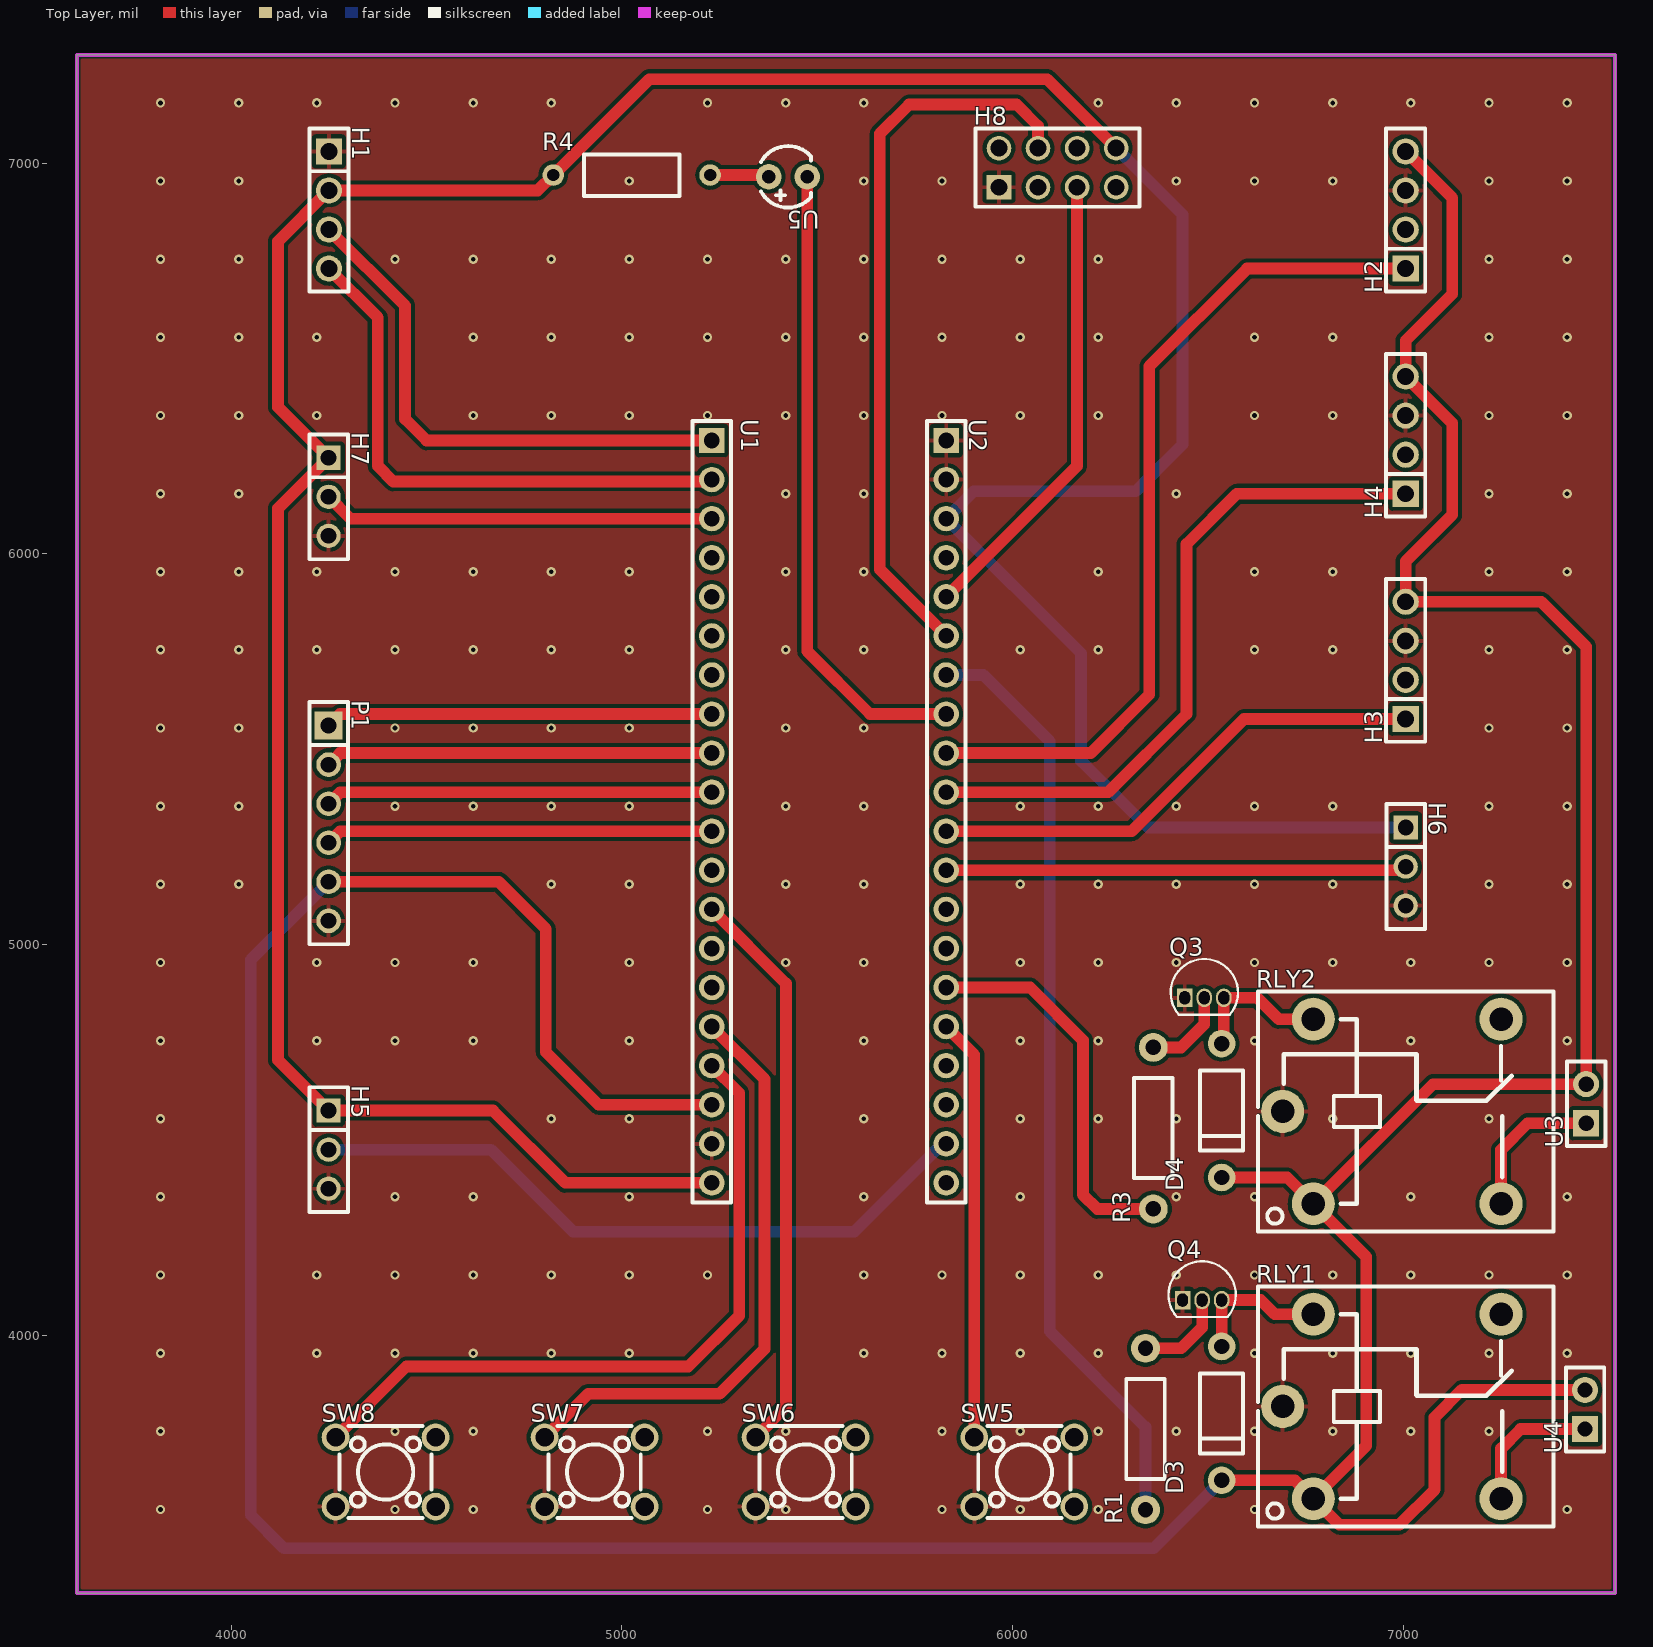
[diagram p0: Top Layer view]
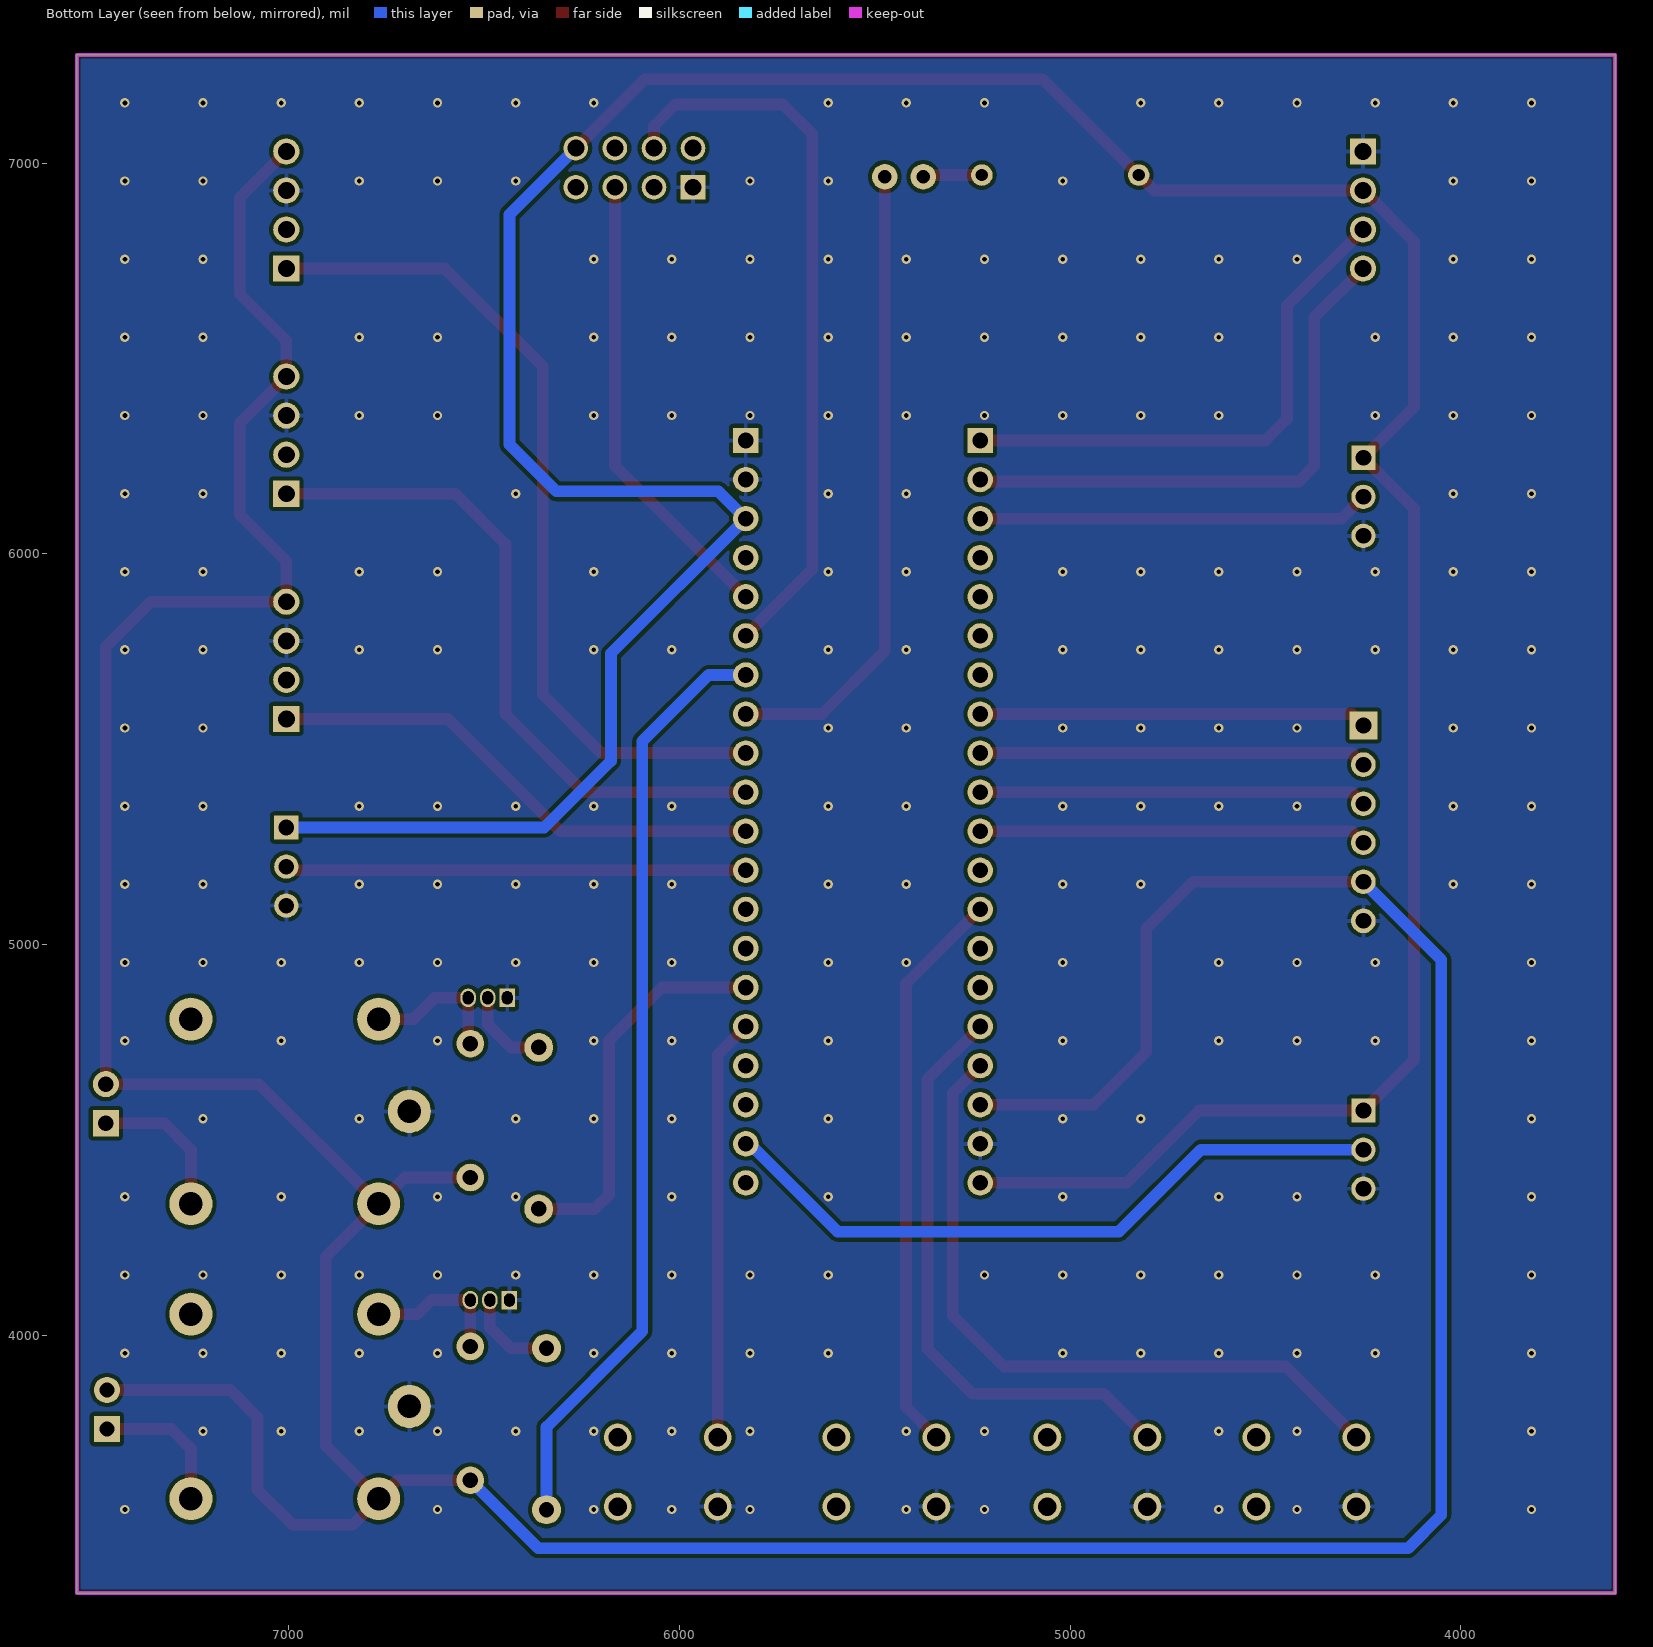
[diagram p1: Bottom Layer view, seen from below]
# Altium PCB MISC51563.pcbdoc
Units mil, origin at the board's own origin, x right, y up, seen from the top; angles counter-clockwise.
Board outline 3937.01 x 3937.01 mil, 2 copper layers (Top Layer, Bottom Layer), stack 62.206 mil thick; 27 components, 38 nets, 127 pads, 246 vias.

## Layer stack, top to bottom
Top Solder Mask Layer: solder mask 0.394, Dk 3.3
Top Layer: signal copper 1.379
Dielectric1: surface 59.449, FR4, Dk 4.5
Bottom Layer: signal copper 1.378
Bottom Solder Mask Layer: solder mask 0.394, Dk 3.3

## Board outline
3605,7277.01 3605,3340 7542.01,3340 7542.01,7277.01

## Design rules (kind name [scope] priority, off if disabled: settings)
BoardOutlineClearance copperThickness2oz_1 [All] p2 off: genericclearance=7.99 ignorepadtopadclearanceinfootprint=FALSE except(0: Arc-SplitContinuation Track-SplitContinuation SMDPad-SplitContinuation THPad-SplitContinuation Via-SplitContinuation Fill-SplitContinuation Region-SplitContinuation Poly-SplitContinuation Text-SplitContinuation Hole-SplitContinuation; 5.98: Arc-CutoutEdge SMDPad-CutoutEdge THPad-CutoutEdge Via-CutoutEdge Fill-CutoutEdge Region-CutoutEdge Text-CutoutEdge; 6.93: Hole-OutlineEdge Hole-CutoutEdge; 10: Poly-OutlineEdge Poly-CutoutEdge; 11.81: Arc-OutlineEdge Track-OutlineEdge SMDPad-OutlineEdge THPad-OutlineEdge Via-OutlineEdge Fill-OutlineEdge Region-OutlineEdge Text-OutlineEdge Track-CutoutEdge)
BoardOutlineClearance Plane_innerPlane_1 [All] p4 off: genericclearance=4.02 ignorepadtopadclearanceinfootprint=FALSE except(0: Arc-SplitContinuation Track-SplitContinuation SMDPad-SplitContinuation THPad-SplitContinuation Via-SplitContinuation Fill-SplitContinuation Region-SplitContinuation Poly-SplitContinuation Text-SplitContinuation Hole-SplitContinuation; 6: SMDPad-CutoutEdge THPad-CutoutEdge Via-CutoutEdge Fill-CutoutEdge Region-CutoutEdge Text-CutoutEdge; 6.93: Hole-OutlineEdge Hole-CutoutEdge; 10: Poly-OutlineEdge Poly-CutoutEdge; 11.8: Arc-OutlineEdge Track-OutlineEdge SMDPad-OutlineEdge THPad-OutlineEdge Via-OutlineEdge Fill-OutlineEdge Region-OutlineEdge Text-OutlineEdge; 11.81: Arc-CutoutEdge Track-CutoutEdge)
BoardOutlineClearance Copper_copperRegion_1 [All] p6 off: genericclearance=4.02 ignorepadtopadclearanceinfootprint=FALSE except(0: Arc-SplitContinuation Track-SplitContinuation SMDPad-SplitContinuation THPad-SplitContinuation Via-SplitContinuation Fill-SplitContinuation Region-SplitContinuation Poly-SplitContinuation Text-SplitContinuation Hole-SplitContinuation; 6: SMDPad-CutoutEdge THPad-CutoutEdge Via-CutoutEdge Fill-CutoutEdge Region-CutoutEdge Text-CutoutEdge; 6.93: Hole-OutlineEdge Hole-CutoutEdge; 10: Poly-OutlineEdge Poly-CutoutEdge; 11.8: Arc-OutlineEdge Track-OutlineEdge SMDPad-OutlineEdge THPad-OutlineEdge Via-OutlineEdge Fill-OutlineEdge Region-OutlineEdge Text-OutlineEdge; 11.81: Arc-CutoutEdge Track-CutoutEdge)
BoardOutlineClearance copperThickness1oz_1 [All] p8: genericclearance=4.02 ignorepadtopadclearanceinfootprint=FALSE except(0: Arc-SplitContinuation Track-SplitContinuation SMDPad-SplitContinuation THPad-SplitContinuation Via-SplitContinuation Fill-SplitContinuation Region-SplitContinuation Poly-SplitContinuation Text-SplitContinuation Hole-SplitContinuation; 6: SMDPad-CutoutEdge THPad-CutoutEdge Via-CutoutEdge Fill-CutoutEdge Region-CutoutEdge Text-CutoutEdge; 6.93: Hole-OutlineEdge Hole-CutoutEdge; 10: Poly-OutlineEdge Poly-CutoutEdge; 11.8: Arc-OutlineEdge Track-OutlineEdge SMDPad-OutlineEdge THPad-OutlineEdge Via-OutlineEdge Fill-OutlineEdge Region-OutlineEdge Text-OutlineEdge; 11.81: Arc-CutoutEdge Track-CutoutEdge)
Clearance copperThickness2oz [All] p1 off: gap=7.99 ignorepadtopadclearanceinfootprint=FALSE except(5.98: SMDPad-Track SMDPad-SMDPad THPad-Track SMDPad-THPad THPad-THPad Track-Via SMDPad-Via THPad-Via Via-Via Fill-Track Region-Track Fill-SMDPad Region-SMDPad Fill-THPad Region-THPad Fill-Via Region-Via Fill-Fill Fill-Region Region-Region Arc-Track Arc-SMDPad Arc-THPad Arc-Via Fill-Arc Region-Arc Arc-Arc Text-Track SMDPad-Text Text-THPad Text-Via Fill-Text Region-Text Arc-Text Text-Text; 6.93: Hole-Track Hole-SMDPad Hole-THPad Hole-Via Fill-Hole Region-Hole Hole-Arc Hole-Text; 10: Poly-Track Poly-SMDPad Poly-THPad Poly-Via Poly-Fill Poly-Region Poly-Poly Poly-Arc Poly-Text Poly-Hole)
Clearance Plane_innerPlane [All] p3 off: gap=4.02 ignorepadtopadclearanceinfootprint=FALSE except(5.98: SMDPad-Track SMDPad-SMDPad THPad-Track SMDPad-THPad THPad-THPad Track-Via SMDPad-Via THPad-Via Via-Via Fill-Track Region-Track Fill-SMDPad Region-SMDPad Fill-THPad Region-THPad Fill-Via Region-Via Fill-Fill Fill-Region Region-Region; 6: Arc-Track Arc-SMDPad Arc-THPad Arc-Via Fill-Arc Region-Arc Arc-Arc Text-Track SMDPad-Text Text-THPad Text-Via Fill-Text Region-Text Arc-Text Text-Text; 6.93: Hole-Track Hole-SMDPad Hole-THPad Hole-Via Fill-Hole Region-Hole Hole-Arc Hole-Text; 10: Poly-Track Poly-SMDPad Poly-THPad Poly-Via Poly-Fill Poly-Region Poly-Poly Poly-Arc Poly-Text Poly-Hole)
Clearance Copper_copperRegion [All] p5 off: gap=4.02 ignorepadtopadclearanceinfootprint=FALSE except(5.98: SMDPad-Track SMDPad-SMDPad THPad-Track SMDPad-THPad THPad-THPad Track-Via SMDPad-Via THPad-Via Via-Via Fill-Track Region-Track Fill-SMDPad Region-SMDPad Fill-THPad Region-THPad Fill-Via Region-Via Fill-Fill Fill-Region Region-Region; 6: Arc-Track Arc-SMDPad Arc-THPad Arc-Via Fill-Arc Region-Arc Arc-Arc Text-Track SMDPad-Text Text-THPad Text-Via Fill-Text Region-Text Arc-Text Text-Text; 6.93: Hole-Track Hole-SMDPad Hole-THPad Hole-Via Fill-Hole Region-Hole Hole-Arc Hole-Text; 10: Poly-Track Poly-SMDPad Poly-THPad Poly-Via Poly-Fill Poly-Region Poly-Poly Poly-Arc Poly-Text Poly-Hole)
Clearance copperThickness1oz [All] p7: gap=4.02 ignorepadtopadclearanceinfootprint=FALSE except(5.98: SMDPad-Track SMDPad-SMDPad THPad-Track SMDPad-THPad THPad-THPad Track-Via SMDPad-Via THPad-Via Via-Via Fill-Track Region-Track Fill-SMDPad Region-SMDPad Fill-THPad Region-THPad Fill-Via Region-Via Fill-Fill Fill-Region Region-Region; 6: Arc-Track Arc-SMDPad Arc-THPad Arc-Via Fill-Arc Region-Arc Arc-Arc Text-Track SMDPad-Text Text-THPad Text-Via Fill-Text Region-Text Arc-Text Text-Text; 6.93: Hole-Track Hole-SMDPad Hole-THPad Hole-Via Fill-Hole Region-Hole Hole-Arc Hole-Text; 10: Poly-Track Poly-SMDPad Poly-THPad Poly-Via Poly-Fill Poly-Region Poly-Poly Poly-Arc Poly-Text Poly-Hole)
DiffPairsRouting differentialPair [All] p1: maxlimit=6 minlimit=6 mostfreqgap=6 toplayer_minwidth=5 toplayer_prefwidth=10 toplayer_maxwidth=100 toplayer_mingap=6 toplayer_prefgap=6 toplayer_maxgap=6 bottomlayer_minwidth=5 bottomlayer_prefwidth=10 bottomlayer_maxwidth=100 bottomlayer_mingap=6 bottomlayer_prefgap=6 bottomlayer_maxgap=6 maxuncoupledlength=10
HoleToHoleClearance otherClearance [All] p1: gap=11.81 allowstackedmicrovias=TRUE
Length netLength [All] p1: minlimit=0 maxlimit=0
PasteMaskExpansion pasteMaskExpansion [All] p1: expansion=0
PlaneConnect innerPlane [All] p1: planeconnectstyle=Relief reliefexpansion=20 reliefentries=4 reliefconductorwidth=10 reliefairgap=10
PolygonConnect copperRegion [All] p1: connectstyle=Relief reliefconductorwidth=10 reliefentries=4 polygonreliefangle="90 Angle" airgapwidth=10 via.connectstyle=Relief via.reliefconductorwidth=10 via.reliefentries=4 via.polygonreliefangle="90 Angle" via.airgapwidth=10
RoutingVias viaSize [All] p1: holewidth=12.01 width=24.02 viastyle="Through Hole" minholewidth=11.81 minwidth=19.68 maxholewidth=248.03 maxwidth=393.7
SolderMaskExpansion solderMaskExpansion [IsVia] p1: expansion=-1000 istentingtop=TRUE
SolderMaskExpansion solderMaskExpansion [All] p2: expansion=2 istentingtop=FALSE
Width copperThickness2oz_2 [All] p1 off: maxlimit=100 minlimit=8 preferedwidth=10
Width copperThickness1oz_2 [All] p2: maxlimit=100 minlimit=5 preferedwidth=10

## Components (designator, comment, footprint, x,y, rotation, side; value= is the part's Value field where it differs from the comment)
D3 "1N4001" DO-41_BD2.4-L4.7-P8.70-D0.9-RD 6535,3800 r90 top
D4 "1N4001" DO-41_BD2.4-L4.7-P8.70-D0.9-RD 6535,4575 r90 top
H1 "oled" HDR-TH_4P-P2.54-V-F 4250,6880 r270 top
H2 "mq2" HDR-TH_4P-P2.54-V-F 7005.98,6880 r90 top
H3 "mq7" HDR-TH_4P-P2.54-V-F 7005.98,5727.36 r90 top
H4 "mq135" HDR-TH_4P-P2.54-V-F 7005.98,6303.68 r90 top
H5 "Buzzer" HDR-TH_3P-P2.54-V-F 4249.21,4475 r270 top
H6 "Photoresistor" HDR-TH_3P-P2.54-V-F 7005.98,5199.47 r270 top
H7 "dht22" HDR-TH_3P-P2.54-V-F 4249.21,6146.05 r270 top
H8 "esp8266" HDR-TH_8P-P2.54-V-F-R2-C4-S2.54 6115,6988.27 r0 top
P1 "uln2003" HDR-TH_6P-P2.54-V-F 4249.21,5310.52 r270 top
Q3 "S8050" TO-92-3_L4.5-W3.5-P1.27-L 6490.51,4863.59 r0 top
Q4 "S8050" TO-92-3_L4.5-W3.5-P1.27-L 6485,4090 r0 top
R1 "1kΩ" RES-TH_BD2.5-L6.5-P10.50-D0.6 6340,3760 r90 top
R3 "1kΩ" RES-TH_BD2.5-L6.5-P10.50-D0.6 6360,4530 r90 top
R4 "10kΩ" RES-TH_BD2.7-L6.2-P10.20-D0.4 5025,6969.41 r0 top
RLY1 "SRD-05VDC-SL-C" RELAY-TH_SRD-XXVDC-XL-C 6970.51,3817.75 r0 top
RLY2 "SRD-05VDC-SL-C" RELAY-TH_SRD-XXVDC-XL-C 6970.51,4572.75 r0 top
SW5 "TC-00104-050E" SW-TH_4P-L6.0-W6.0-P4.50-LS6.5 6030,3650 r0 top
SW6 "TC-00104-050E" SW-TH_4P-L6.0-W6.0-P4.50-LS6.5 5470,3650 r0 top
SW7 "TC-00104-050E" SW-TH_4P-L6.0-W6.0-P4.50-LS6.5 4930,3650 r0 top
SW8 "TC-00104-050E" SW-TH_4P-L6.0-W6.0-P4.50-LS6.5 4395,3650 r0 top
U1 "KH-2.54FH-1X20P-H8.5" HDR-TH_20P-P2.54-V-F-2 5230,5340 r270 top
U2 "KH-2.54FH-1X20P-H8.5" HDR-TH_20P-P2.54-V-F-2 5830,5340 r270 top
U3 "Humidifier" HDR-TH_2P-P2.54-V-F 7467.83,4592.75 r90 top
U4 "Fan" HDR-TH_2P-P2.54-V-F 7465,3810 r90 top
U5 "204-10SDRD/S530-A3/F182-68" LED-TH_BD4.0-P2.50-RD 5425,6965 r180 top

## Footprints (in the part's own frame and the unit in brackets; to place one, negate y for a bottom-side part, rotate by r counter-clockwise, add the part's x,y. Pads: shape width x height; smd on the part's side, far side on the other; paste and mask are expansions set on the pad)
DO-41_BD2.4-L4.7-P8.70-D0.9-RD [mm]
  round 1.8 hole 1: 1(-4.35,0) 2(4.35,0)
  silkscreen extent -2.6,-1.4 2.6,1.4
HDR-TH_2P-P2.54-V-F [mm]
  rect 1.7x1.7 hole 1: 1(-1.27,0)
  round 1.7 hole 1: 2(1.27,0)
  silkscreen extent -2.74,-1.25 2.74,1.25
HDR-TH_3P-P2.54-V-F [mil]
  rect 62x62 hole 40.16: 1(-100,0)
  round 62 hole 40.16: 2(0,0) 3(100,0)
  silkscreen extent -160,-49 160,49
HDR-TH_4P-P2.54-V-F [mm]
  rect 1.7x1.7 hole 1.1: 1(-3.81,0)
  round 1.7 hole 1.1: 2(-1.27,0) 3(1.27,0) 4(3.81,0)
  silkscreen extent -5.29,-1.27 5.29,1.27
HDR-TH_6P-P2.54-V-F [mm]
  rect 1.8x1.8 hole 1.02: 1(-6.35,0)
  round 1.6 hole 1.02: 2(-3.81,0) 3(-1.27,0) 4(1.27,0) 5(3.81,0) 6(6.35,0)
  silkscreen extent -7.87,-1.25 7.87,1.25
HDR-TH_8P-P2.54-V-F-R2-C4-S2.54 [mm]
  rect 1.6x1.6 hole 1.1: 1(-3.81,-1.27)
  round 1.6 hole 1.1: 2(-3.81,1.27) 3(-1.27,-1.27) 4(-1.27,1.27) 5(1.27,-1.27) 6(1.27,1.27) 7(3.81,-1.27) 8(3.81,1.27)
  silkscreen extent -5.33,-2.54 5.33,2.54
HDR-TH_20P-P2.54-V-F-2 [mm]
  rect 1.65x1.65 hole 1.02: 1(-24.13,0)
  round 1.65 hole 1.02: 2(-21.59,0) 3(-19.05,0) 4(-16.51,0) 5(-13.97,0) 6(-11.43,0) 7(-8.89,0) 8(-6.35,0) 9(-3.81,0) 10(-1.27,0) 11(1.27,0) 12(3.81,0) 13(6.35,0) 14(8.89,0) 15(11.43,0) 16(13.97,0) 17(16.51,0) 18(19.05,0) 19(21.59,0) 20(24.13,0)
  silkscreen extent -25.4,-1.25 25.4,1.25
LED-TH_BD4.0-P2.50-RD [mil]
  round 65 hole 35.43: 1(-49.21,0) 2(49.22,0)
  silkscreen extent -59,-79 69,79
RELAY-TH_SRD-XXVDC-XL-C [mil]
  round 110 hole 60: 1(-200.79,-236.22) 2(279.53,-236.2) 3(279.53,236.2) 4(-200.79,236.22) 5(-279.53,0)
  silkscreen extent -342,-307 413,307
RES-TH_BD2.5-L6.5-P10.50-D0.6 [mil]
  round 74 hole 39.37: 1(-206.69,0) 2(206.69,0)
  silkscreen extent -128,-49 128,49
RES-TH_BD2.7-L6.2-P10.20-D0.4 [mm]
  round 1.4 hole 0.8 copper offset 0,0: 1(-5.1,0) 2(5.1,0)
  silkscreen extent -3.1,-1.35 3.1,1.35
SW-TH_4P-L6.0-W6.0-P4.50-LS6.5 [mm]
  round 1.8 hole 1.2: 1(-3.25,2.25) 2(3.25,2.25) 3(-3.25,-2.25) 4(3.25,-2.25)
  silkscreen extent -3,-3 3,3
TO-92-3_L4.5-W3.5-P1.27-L [mm]
  rect 1x1.2 hole 0.7 slot 0.85 at 90 deg: 1(-1.27,0)
  oval 1x1.2 hole 0.7 slot 0.85 at 90 deg: 2(0,0) 3(1.27,0)
  silkscreen extent -2.19,-1.1 2.19,2.52

## Via types
v1: diameter 24.02, hole 12, Top Layer to Bottom Layer, 246 vias

## Nets (pads, with @x,y where several pads share a name; then routed paths per layer and width w, separated by ;. In a path a pad name is that pad's centre, name@x,y a point inside that pad or via, vN(x,y) a via of type N, cw(c..) or ccw(c..) an arc to the next point about the centre after c; other vN are vias at no path point)
$1N3: R4.2 U5.2 | length 151.8
  Top Layer w30: R4.2 5371.38,6969.41 U5.2
$1N5: SW7.2
$1N6: SW6.2
$1N12: RLY2.2 U3.1 | length 384.3
  Top Layer w30: RLY2.2 7250.04,4475.04 7317.75,4542.75 U3.1
$1N16: Q3.2 R3.2 | length 222.9
  Top Layer w30: R3.2 6431.69,4736.69 6490.51,4795.51 Q3.2
$1N17: D4.2 Q3.3 RLY2.4 | length 371.4
  Top Layer w30: D4.2 6540.51,4751.77 Q3.3 6626.41,4863.59 6681.03,4808.97 RLY2.4
$1N18: RLY1.2 U4.1 | length 364.1
  Top Layer w30: RLY1.2 7250.04,3710.04 7300,3760 U4.1
$1N22: Q4.2 R1.2 | length 237.1
  Top Layer w30: R1.2 6431.69,3966.69 6485,4020 Q4.2
$1N23: D3.2 Q4.3 RLY1.4 | length 368.4
  Top Layer w30: D3.2 Q4.3 6635,4090 6671.03,4053.97 RLY1.4
$1N97: SW8.2
+5V: D3.1 D4.1 H2.4 H3.4 H4.4 P1.5 RLY1.1 RLY2.1 U1.18 U3.2 U4.2 | length 11858.6
  Top Layer w30: P1.5 4684.48,5160.52 4805,5040 4805,4725 4940,4590 U1.18 ; D3.1 6722.51,3628.74 RLY1.1 ; D4.1 6702.51,4403.74 RLY2.1 ; H2.4 7125,6910.98 7125,6665 7005.98,6545.98 H4.4 7125,6334.66 7125,6100 7005.98,5980.98 H3.4 7352.64,5877.36 7467.83,5762.17 U3.2 7075.94,4642.75 RLY2.1 ; U4.2 7150,3860 7080,3790 7080,3605 6990,3515 6836.25,3515 RLY1.1 ; RLY1.1 6905,3716.82 6905,4201.25 RLY2.1
  Bottom Layer w30: P1.5 4050,4961.31 4050,3540 4135,3455 6361.26,3455 D3.1
GND: H1.1 H2.3 H3.3 H4.3 H5.3 H6.3 H7.3 H8.1 P1.6 Q3.1 Q4.1 RLY1.5 RLY2.5 SW5.3 SW6.3 SW7.3 SW8.3 U1.19 U2.1 U2.2
  other v1: 3819.1,3554.1 4419.1,3554.1 4619.1,3554.1 5219.1,3554.1 5419.1,3554.1 5819.1,3554.1 6019.1,3554.1 6219.1,3554.1 6619.1,3554.1 7419.1,3554.1 3819.1,3754.1 4419.1,3754.1 4619.1,3754.1 5219.1,3754.1 5419.1,3754.1 5819.1,3754.1 6019.1,3754.1 6219.1,3754.1 6419.1,3754.1 6619.1,3754.1 6819.1,3754.1 7019.1,3754.1 7219.1,3754.1 3819.1,3954.1 4219.1,3954.1 4419.1,3954.1 4619.1,3954.1 4819.1,3954.1 5019.1,3954.1 5619.1,3954.1 5819.1,3954.1 6019.1,3954.1 6219.1,3954.1 6619.1,3954.1 6819.1,3954.1 7019.1,3954.1 7219.1,3954.1 7419.1,3954.1 3819.1,4154.1 4219.1,4154.1 4419.1,4154.1 4619.1,4154.1 4819.1,4154.1 5019.1,4154.1 5219.1,4154.1 5619.1,4154.1 5819.1,4154.1 6019.1,4154.1 6219.1,4154.1 6419.1,4154.1 6619.1,4154.1 6819.1,4154.1 7019.1,4154.1 7219.1,4154.1 7419.1,4154.1 3819.1,4354.1 4419.1,4354.1 4619.1,4354.1 5019.1,4354.1 5619.1,4354.1 6019.1,4354.1 6419.1,4354.1 6619.1,4354.1 7019.1,4354.1 7419.1,4354.1 3819.1,4554.1 4819.1,4554.1 5019.1,4554.1 5619.1,4554.1 6019.1,4554.1 6219.1,4554.1 6419.1,4554.1 6819.1,4554.1 7219.1,4554.1 3819.1,4754.1 4219.1,4754.1 4419.1,4754.1 4619.1,4754.1 5019.1,4754.1 5619.1,4754.1 6019.1,4754.1 6219.1,4754.1 6619.1,4754.1 7019.1,4754.1 7419.1,4754.1 3819.1,4954.1 4219.1,4954.1 4419.1,4954.1 4619.1,4954.1 5019.1,4954.1 5419.1,4954.1 5619.1,4954.1 6019.1,4954.1 6219.1,4954.1 6419.1,4954.1 6619.1,4954.1 6819.1,4954.1 7019.1,4954.1 7219.1,4954.1 7419.1,4954.1 3819.1,5154.1 4019.1,5154.1 4819.1,5154.1 5019.1,5154.1 5419.1,5154.1 5619.1,5154.1 6019.1,5154.1 6219.1,5154.1 6419.1,5154.1 6619.1,5154.1 6819.1,5154.1 7219.1,5154.1 7419.1,5154.1 3819.1,5354.1 4019.1,5354.1 4419.1,5354.1 4619.1,5354.1 4819.1,5354.1 5019.1,5354.1 5419.1,5354.1 5619.1,5354.1 6019.1,5354.1 6219.1,5354.1 6419.1,5354.1 6619.1,5354.1 6819.1,5354.1 7219.1,5354.1 7419.1,5354.1 3819.1,5554.1 4019.1,5554.1 4419.1,5554.1 4619.1,5554.1 4819.1,5554.1 5019.1,5554.1 5419.1,5554.1 5619.1,5554.1 7219.1,5554.1 7419.1,5554.1 3819.1,5754.1 4019.1,5754.1 4219.1,5754.1 4419.1,5754.1 4619.1,5754.1 4819.1,5754.1 5019.1,5754.1 5419.1,5754.1 5619.1,5754.1 6019.1,5754.1 6219.1,5754.1 6619.1,5754.1 6819.1,5754.1 7219.1,5754.1 7419.1,5754.1 3819.1,5954.1 4019.1,5954.1 4219.1,5954.1 4419.1,5954.1 4619.1,5954.1 4819.1,5954.1 5019.1,5954.1 5419.1,5954.1 5619.1,5954.1 6219.1,5954.1 6619.1,5954.1 6819.1,5954.1 7219.1,5954.1 7419.1,5954.1 3819.1,6154.1 4019.1,6154.1 5419.1,6154.1 5619.1,6154.1 6419.1,6154.1 7219.1,6154.1 7419.1,6154.1 3819.1,6354.1 4019.1,6354.1 4219.1,6354.1 4619.1,6354.1 4819.1,6354.1 5019.1,6354.1 5219.1,6354.1 5419.1,6354.1 5619.1,6354.1 5819.1,6354.1 6019.1,6354.1 6219.1,6354.1 6619.1,6354.1 6819.1,6354.1 7219.1,6354.1 7419.1,6354.1 3819.1,6554.1 4019.1,6554.1 4219.1,6554.1 4619.1,6554.1 4819.1,6554.1 5019.1,6554.1 5219.1,6554.1 5419.1,6554.1 5619.1,6554.1 5819.1,6554.1 6019.1,6554.1 6219.1,6554.1 6619.1,6554.1 6819.1,6554.1 7219.1,6554.1 7419.1,6554.1 3819.1,6754.1 4019.1,6754.1 4419.1,6754.1 4619.1,6754.1 4819.1,6754.1 5019.1,6754.1 5219.1,6754.1 5419.1,6754.1 5619.1,6754.1 5819.1,6754.1 6019.1,6754.1 6219.1,6754.1 7219.1,6754.1 7419.1,6754.1 3819.1,6954.1 4019.1,6954.1 5019.1,6954.1 5619.1,6954.1 5819.1,6954.1 6419.1,6954.1 6619.1,6954.1 6819.1,6954.1 7219.1,6954.1 7419.1,6954.1 3819.1,7154.1 4019.1,7154.1 4219.1,7154.1 4419.1,7154.1 4619.1,7154.1 4819.1,7154.1 5219.1,7154.1 5419.1,7154.1 5619.1,7154.1 6219.1,7154.1 6419.1,7154.1 6619.1,7154.1 6819.1,7154.1 7019.1,7154.1 7219.1,7154.1 7419.1,7154.1
PA0: SW5.1 U2.16 | length 1081.3
  Top Layer w30: U2.16 5902.05,4717.95 SW5.1
PA1: R3.1 U2.15 | length 996.1
  Top Layer w30: U2.15 6045,4890 6180,4755 6180,4360 6216.69,4323.31 R3.1
PA4: H6.2 U2.12 | length 1179.9
  Top Layer w30: U2.12 6996.51,5190 H6.2
PA5: H3.1 U2.11 | length 1295
  Top Layer w30: U2.11 6305,5290 6592.36,5577.36 H3.1
PA6: H4.1 U2.10 | length 1747.1
  Top Layer w30: U2.10 6245,5390 6445,5590 6445,6025 6573.68,6153.68 H4.1
PA7: H2.1 U2.9 | length 2181.7
  Top Layer w30: U2.9 6200,5490 6350,5640 6350,6480 6600,6730 H2.1
PA8: U1.5
PA9: U1.6
PA11: P1.1 U1.8 | length 993
  Top Layer w30: P1.1 4278.69,5590 U1.8
PA12: P1.2 U1.9 | length 993
  Top Layer w30: P1.2 4278.69,5490 U1.9
PA15: P1.3 U1.10 | length 993
  Top Layer w30: P1.3 4278.69,5390 U1.10
PB0: U2.8 U5.1 | length 1636.6
  Top Layer w30: U5.1 5474.21,5750.79 5635,5590 U2.8
PB1: R1.1 U2.7 | length 2403.6
  Bottom Layer w30: U2.7 5925,5690 6095,5520 6095,4010 6340,3765 R1.1
PB3: P1.4 U1.11 | length 993
  Top Layer w30: P1.4 4278.69,5290 U1.11
PB5: SW6.1 U1.13 | length 1462.4
  Top Layer w30: U1.13 5420,4900 5420,3816.53 SW6.1
PB6: U1.14
PB7: U1.15
PB8: SW7.1 U1.16 | length 1537.7
  Top Layer w30: SW7.1 4913.47,3850 5250,3850 5365,3965 5365,4655 U1.16
PB9: SW8.1 U1.17 | length 1830.9
  Top Layer w30: SW8.1 4448.47,3920 5170,3920 5300,4050 5300,4620 U1.17
PB10: H8.4 U2.6 | length 1871
  Top Layer w30: U2.6 5660,5960 5660,7075 5735,7150 6010,7150 6065,7095 H8.4
PB11: H8.5 U2.5 | length 1187
  Top Layer w30: U2.5 6165,6225 H8.5
PB12: H1.3 U1.1 | length 1373.6
  Top Layer w30: H1.3 4445,6635 4445,6345 4500,6290 U1.1
PB13: H1.4 U1.2 | length 1430.4
  Top Layer w30: H1.4 4375,6605 4375,6225 4415,6185 5225,6185 U1.2
PB14: H7.2 U1.3 | length 1004
  Top Layer w30: H7.2 4305.26,6090 U1.3
PC13: H5.2 U2.19 | length 1761
  Bottom Layer w30: H5.2 4665,4475 4875,4265 5595,4265 5820,4490 U2.19
VCC: H1.2 H5.1 H6.1 H7.1 H8.8 R4.1 U1.20 U2.3 | length 9010
  Top Layer w30: U1.20 4855,4390 4670,4575 H5.1 4120,4704.21 4120,6116.84 H7.1 4120,6375.26 4120,6800 H1.2 4784.8,6930 R4.1 5069.8,7215 6088.27,7215 H8.8
  Bottom Layer w30: H8.8 6435,6868.27 6435,6280 6315,6160 5900,6160 U2.3 6175,5745 6175,5470 6345.53,5299.47 H6.1
pads on no net: H2.2 H3.2 H4.2 H8.2 H8.3 H8.6 H8.7 RLY1.3 RLY2.3 SW5.2 SW5.4 SW6.4 SW7.4 SW8.4 U1.4 U1.7 U1.12 U2.4 U2.13 U2.14 U2.17 U2.18 U2.20

## Polygon pours and split planes (outlines as drawn)
GND on Top Layer (solid, remove dead copper, pour order 8): 3400,7355 3400,3115 8100,3115 8100,7355
GND on Bottom Layer (solid, remove dead copper, pour order 12): 3000,7630 3000,3000 8465,3000 8465,7630

## Keep-outs
Board Outline Layer:
  the board outline again, w10